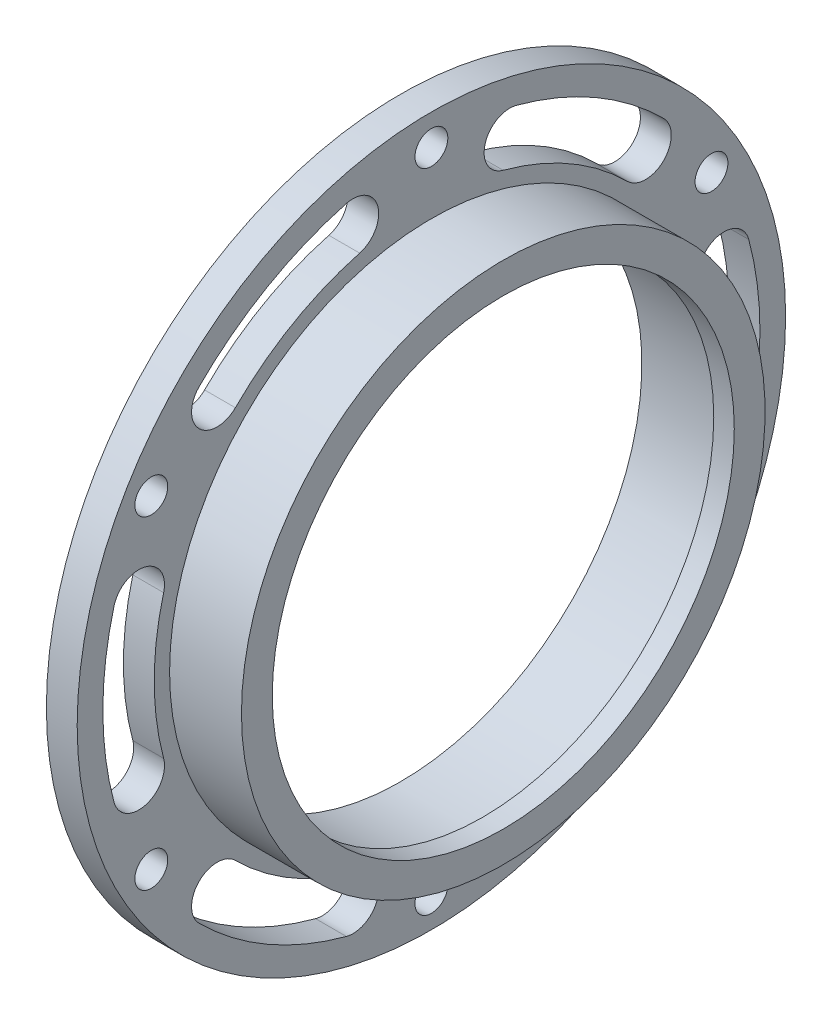
SolidWorks part; units mm, degrees
material "6061 合金"
ref_plane "前视基准面" through (0, 0, 0) normal (0, 0, 1) x (1, 0, 0)
ref_plane "上视基准面" through (0, 0, 0) normal (0, 1, 0) x (1, 0, 0)
ref_plane "右视基准面" through (0, 0, 0) normal (1, 0, 0) x (0, 0, -1)
other "Configuration Table"
sketch "草图1" plane through (0, 0, 0) normal (0, 1, 0) x (1, 0, 0)
  line L0 (-505.7965, 0) -> (24784.028, 0) construction
  line L1 (0, 23.5) -> (0, 34.5)
  line L2 (0, 34.5) -> (3, 34.5)
  line L3 (3, 34.5) -> (3, 25.5)
  line L4 (3, 25.5) -> (10, 25.5)
  line L5 (10, 25.5) -> (10, 22.5)
  line L6 (10, 22.5) -> (8, 22.5)
  line L7 (8, 22.5) -> (8, 23.5)
  line L8 (8, 23.5) -> (0, 23.5)
  dimension "D1" = 47
  dimension "D2" = 51
  dimension "D3" = 69
  dimension "D4" = 8
  dimension "D5" = 3
  dimension "D6" = 1
  dimension "D7" = 2
revolve "旋转1" add sketch "草图1" angle 360 about L0
sketch "草图2" plane through (3, 0, 0) normal (1, 0, 0) x (0, 0, -1)
  circle A1 centre (0, 0) radius 31.5 construction
  circle A2 centre (0, 31.5) radius 1.6
  circle A3 centre (27.2798, 15.75) radius 1.6
  circle A4 centre (27.2798, -15.75) radius 1.6
  circle A5 centre (0, -31.5) radius 1.6
  circle A6 centre (-27.2798, -15.75) radius 1.6
  circle A7 centre (-27.2798, 15.75) radius 1.6
  circle A8 centre (0, 0) radius 28.5 construction
  point P17 (0, 0)
  dimension "D1" = 63
  dimension "D2" = 3.2
  dimension "D4" = 57
  dimension "D3" = 6
extrude "切除-拉伸1" cut sketch "草图2" against normal through all
sketch "草图3" plane through (3, 0, 0) normal (1, 0, 0) x (0, 0, -1)
  line L0 (7.6352, 28.4948) -> (0, 0) construction
  line L1 (0, 0) -> (20.8597, 20.8597) construction
  line L2 (14.75, 25.5477) -> (0, 0) construction
  line L3 (0, 0) -> (0, 31.5) construction
  circle A0 centre (0, 0) radius 29.5 construction
  arc A1 (7.6352, 28.4948) -> (20.8597, 20.8597) centre (0, 0) cw construction
  arc A2 (22.6274, 22.6274) -> (8.2822, 30.9096) centre (0, 0) ccw
  arc A3 (19.0919, 19.0919) -> (6.9881, 26.08) centre (0, 0) ccw
  arc A4 (19.0919, 19.0919) -> (22.6274, 22.6274) centre (20.8597, 20.8597) ccw
  arc A5 (8.2822, 30.9096) -> (6.9881, 26.08) centre (7.6352, 28.4948) ccw
  arc A6 (28.4948, 7.6352) -> (28.4948, -7.6352) centre (0, 0) cw construction
  arc A7 (30.9096, -8.2822) -> (30.9096, 8.2822) centre (0, 0) ccw
  arc A8 (26.08, -6.9881) -> (26.08, 6.9881) centre (0, 0) ccw
  arc A9 (26.08, -6.9881) -> (30.9096, -8.2822) centre (28.4948, -7.6352) ccw
  arc A10 (30.9096, 8.2822) -> (26.08, 6.9881) centre (28.4948, 7.6352) ccw
  arc A11 (20.8597, -20.8597) -> (7.6352, -28.4948) centre (0, 0) cw construction
  arc A12 (8.2822, -30.9096) -> (22.6274, -22.6274) centre (0, 0) ccw
  arc A13 (6.9881, -26.08) -> (19.0919, -19.0919) centre (0, 0) ccw
  arc A14 (6.9881, -26.08) -> (8.2822, -30.9096) centre (7.6352, -28.4948) ccw
  arc A15 (22.6274, -22.6274) -> (19.0919, -19.0919) centre (20.8597, -20.8597) ccw
  arc A16 (-7.6352, -28.4948) -> (-20.8597, -20.8597) centre (0, 0) cw construction
  arc A17 (-22.6274, -22.6274) -> (-8.2822, -30.9096) centre (0, 0) ccw
  arc A18 (-19.0919, -19.0919) -> (-6.9881, -26.08) centre (0, 0) ccw
  arc A19 (-19.0919, -19.0919) -> (-22.6274, -22.6274) centre (-20.8597, -20.8597) ccw
  arc A20 (-8.2822, -30.9096) -> (-6.9881, -26.08) centre (-7.6352, -28.4948) ccw
  arc A21 (-28.4948, -7.6352) -> (-28.4948, 7.6352) centre (0, 0) cw construction
  arc A22 (-30.9096, 8.2822) -> (-30.9096, -8.2822) centre (0, 0) ccw
  arc A23 (-26.08, 6.9881) -> (-26.08, -6.9881) centre (0, 0) ccw
  arc A24 (-26.08, 6.9881) -> (-30.9096, 8.2822) centre (-28.4948, 7.6352) ccw
  arc A25 (-30.9096, -8.2822) -> (-26.08, -6.9881) centre (-28.4948, -7.6352) ccw
  arc A26 (-20.8597, 20.8597) -> (-7.6352, 28.4948) centre (0, 0) cw construction
  arc A27 (-8.2822, 30.9096) -> (-22.6274, 22.6274) centre (0, 0) ccw
  arc A28 (-6.9881, 26.08) -> (-19.0919, 19.0919) centre (0, 0) ccw
  arc A29 (-6.9881, 26.08) -> (-8.2822, 30.9096) centre (-7.6352, 28.4948) ccw
  arc A30 (-22.6274, 22.6274) -> (-19.0919, 19.0919) centre (-20.8597, 20.8597) ccw
  point P5 (14.75, 25.5477)
  point P20 (29.5, 0)
  point P27 (14.75, -25.5477)
  point P34 (-14.75, -25.5477)
  point P41 (-29.5, 0)
  point P48 (-14.75, 25.5477)
  point P53 (0, 0)
  dimension "D1" = 59
  dimension "D2" = 5
  dimension "D5" = 6
  dimension "D3" = 30
  dimension "D4" = 30
extrude "切除-拉伸2" cut sketch "草图3" against normal through all
